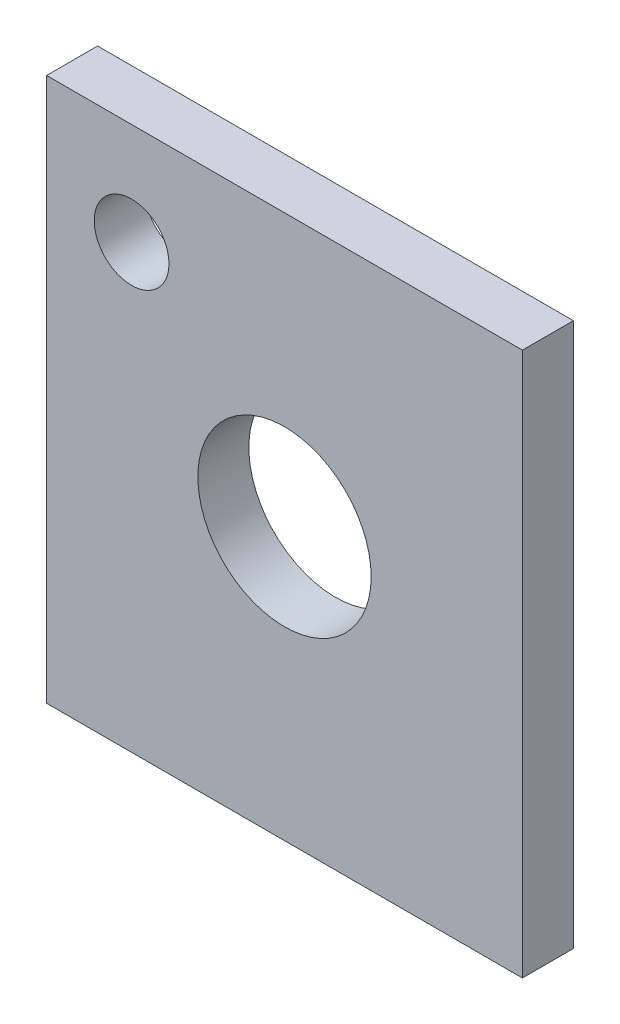
from build123d import *

# Parameters (mm, degrees)
SKETCH_1_W          = 28
SKETCH_1_H          = 32
EXTRUDE_1_DEPTH     = 1.5
SKETCH_2_R          = 5.1
SKETCH_2_R_2        = 2.2
CUT_EXTRUDE_1_DEPTH = 11.5


with BuildPart() as part:
    # 草图1 → 凸台-拉伸1 (new, symmetric)
    with BuildSketch(Plane.XY):
        Rectangle(SKETCH_1_W, SKETCH_1_H)
    extrude(amount=EXTRUDE_1_DEPTH, both=True)

    # 草图2 → 切除-拉伸1 (cut, symmetric)
    with BuildSketch(Plane.XY):
        Circle(SKETCH_2_R)
        with Locations((-9, 10)):
            Circle(SKETCH_2_R_2)
    extrude(amount=CUT_EXTRUDE_1_DEPTH, both=True, mode=Mode.SUBTRACT)


solid = part.part
